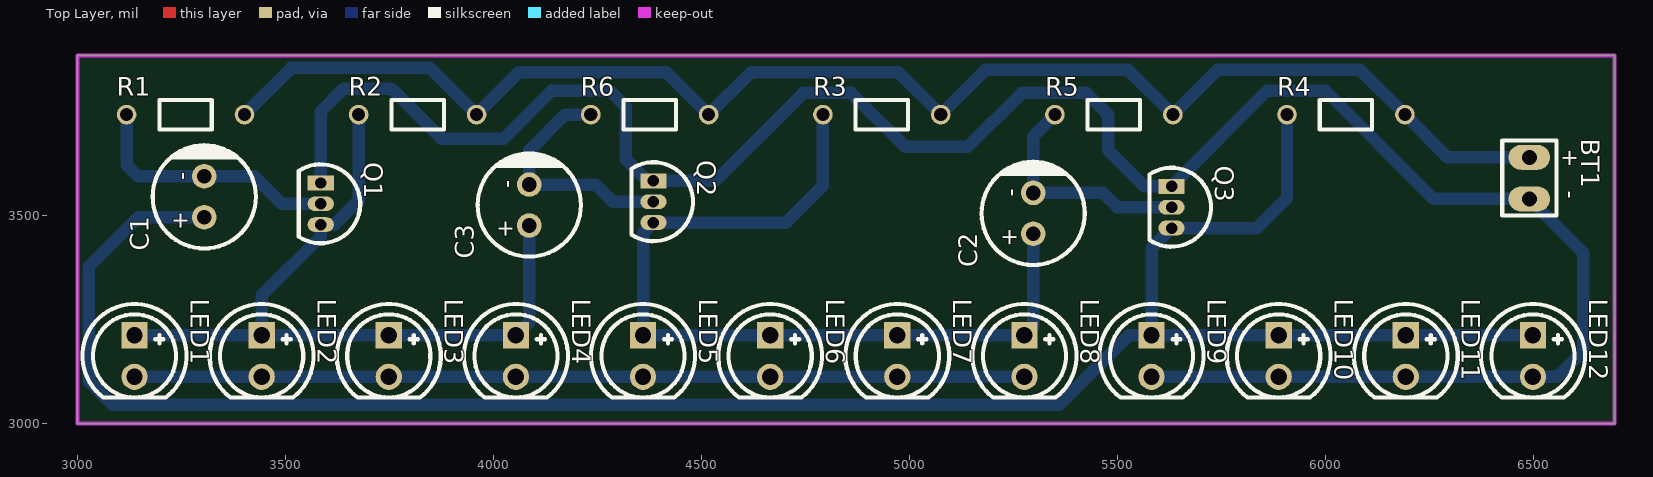
[diagram p0: Top Layer view]
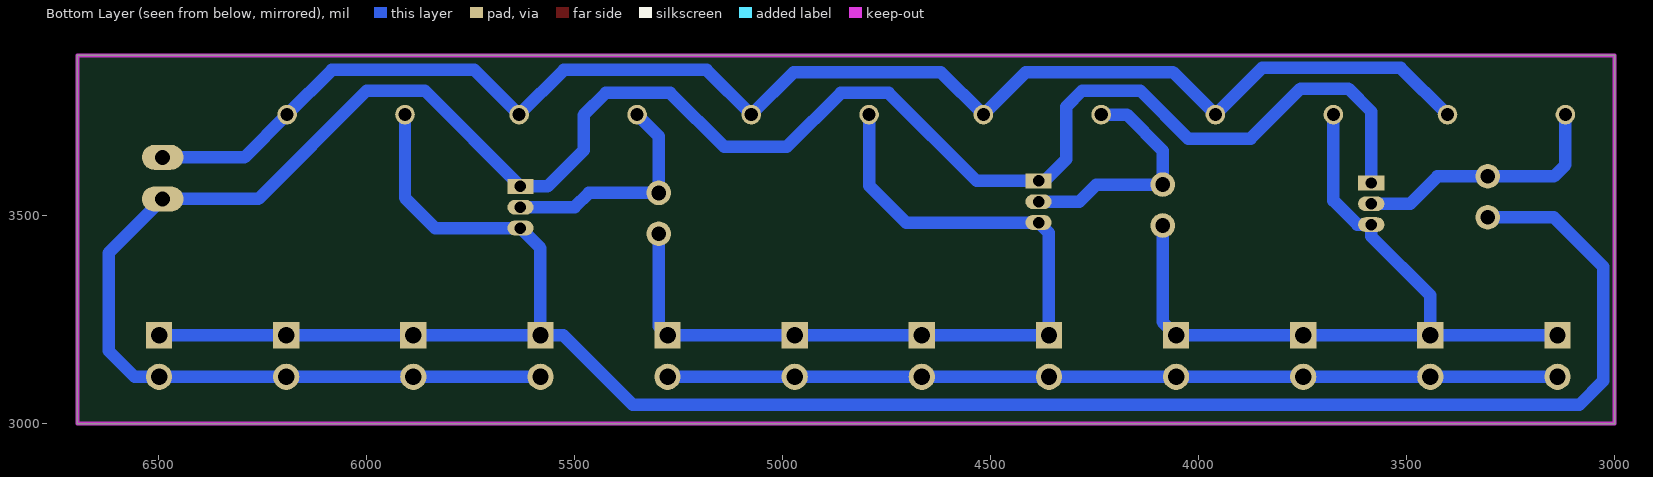
[diagram p1: Bottom Layer view, seen from below]
# Altium PCB MISC75405.pcbdoc
Units mil, origin at the board's own origin, x right, y up, seen from the top; angles counter-clockwise.
Board outline 3695 x 885 mil, 2 copper layers (Top Layer, Bottom Layer), stack 62.206 mil thick; 25 components, 8 nets, 53 pads, 0 vias.

## Layer stack, top to bottom
Top Solder Mask Layer: solder mask 0.394, Dk 3.3
Top Layer: signal copper 1.379
Dielectric1: surface 59.449, FR4, Dk 4.5
Bottom Layer: signal copper 1.378
Bottom Solder Mask Layer: solder mask 0.394, Dk 3.3

## Board outline
3000,3885 3000,3000 6695,3000 6695,3885

## Design rules (kind name [scope] priority, off if disabled: settings)
BoardOutlineClearance copperThickness2oz_1 [All] p2 off: genericclearance=7.99 ignorepadtopadclearanceinfootprint=FALSE except(0: Arc-SplitContinuation Track-SplitContinuation SMDPad-SplitContinuation THPad-SplitContinuation Via-SplitContinuation Fill-SplitContinuation Region-SplitContinuation Poly-SplitContinuation Text-SplitContinuation Hole-SplitContinuation; 5.98: Arc-CutoutEdge SMDPad-CutoutEdge THPad-CutoutEdge Via-CutoutEdge Fill-CutoutEdge Region-CutoutEdge Text-CutoutEdge; 6.93: Hole-OutlineEdge Hole-CutoutEdge; 10: Poly-OutlineEdge Poly-CutoutEdge; 11.81: Arc-OutlineEdge Track-OutlineEdge SMDPad-OutlineEdge THPad-OutlineEdge Via-OutlineEdge Fill-OutlineEdge Region-OutlineEdge Text-OutlineEdge Track-CutoutEdge)
BoardOutlineClearance copperThickness1oz_1 [All] p4: genericclearance=4.02 ignorepadtopadclearanceinfootprint=FALSE except(0: Arc-SplitContinuation Track-SplitContinuation SMDPad-SplitContinuation THPad-SplitContinuation Via-SplitContinuation Fill-SplitContinuation Region-SplitContinuation Poly-SplitContinuation Text-SplitContinuation Hole-SplitContinuation; 6: SMDPad-CutoutEdge THPad-CutoutEdge Via-CutoutEdge Fill-CutoutEdge Region-CutoutEdge Text-CutoutEdge; 6.93: Hole-OutlineEdge Hole-CutoutEdge; 10: Poly-OutlineEdge Poly-CutoutEdge; 11.8: Arc-OutlineEdge Track-OutlineEdge SMDPad-OutlineEdge THPad-OutlineEdge Via-OutlineEdge Fill-OutlineEdge Region-OutlineEdge Text-OutlineEdge; 11.81: Arc-CutoutEdge Track-CutoutEdge)
Clearance copperThickness2oz [All] p1 off: gap=7.99 ignorepadtopadclearanceinfootprint=FALSE except(5.98: SMDPad-Track SMDPad-SMDPad THPad-Track SMDPad-THPad THPad-THPad Track-Via SMDPad-Via THPad-Via Via-Via Fill-Track Region-Track Fill-SMDPad Region-SMDPad Fill-THPad Region-THPad Fill-Via Region-Via Fill-Fill Fill-Region Region-Region Arc-Track Arc-SMDPad Arc-THPad Arc-Via Fill-Arc Region-Arc Arc-Arc Text-Track SMDPad-Text Text-THPad Text-Via Fill-Text Region-Text Arc-Text Text-Text; 6.93: Hole-Track Hole-SMDPad Hole-THPad Hole-Via Fill-Hole Region-Hole Hole-Arc Hole-Text; 10: Poly-Track Poly-SMDPad Poly-THPad Poly-Via Poly-Fill Poly-Region Poly-Poly Poly-Arc Poly-Text Poly-Hole)
Clearance copperThickness1oz [All] p3: gap=4.02 ignorepadtopadclearanceinfootprint=FALSE except(5.98: SMDPad-Track SMDPad-SMDPad THPad-Track SMDPad-THPad THPad-THPad Track-Via SMDPad-Via THPad-Via Via-Via Fill-Track Region-Track Fill-SMDPad Region-SMDPad Fill-THPad Region-THPad Fill-Via Region-Via Fill-Fill Fill-Region Region-Region; 6: Arc-Track Arc-SMDPad Arc-THPad Arc-Via Fill-Arc Region-Arc Arc-Arc Text-Track SMDPad-Text Text-THPad Text-Via Fill-Text Region-Text Arc-Text Text-Text; 6.93: Hole-Track Hole-SMDPad Hole-THPad Hole-Via Fill-Hole Region-Hole Hole-Arc Hole-Text; 10: Poly-Track Poly-SMDPad Poly-THPad Poly-Via Poly-Fill Poly-Region Poly-Poly Poly-Arc Poly-Text Poly-Hole)
DiffPairsRouting differentialPair [All] p1: maxlimit=6 minlimit=6 mostfreqgap=6 toplayer_minwidth=5 toplayer_prefwidth=10 toplayer_maxwidth=100 toplayer_mingap=6 toplayer_prefgap=6 toplayer_maxgap=6 bottomlayer_minwidth=5 bottomlayer_prefwidth=10 bottomlayer_maxwidth=100 bottomlayer_mingap=6 bottomlayer_prefgap=6 bottomlayer_maxgap=6 maxuncoupledlength=10
HoleToHoleClearance otherClearance [All] p1: gap=11.81 allowstackedmicrovias=TRUE
Length netLength [All] p1: minlimit=0 maxlimit=0
MatchedLengths netLengthTolerance [All] p1: tolerance=1000
PasteMaskExpansion pasteMaskExpansion [All] p1: expansion=0
PlaneConnect innerPlane [All] p1: planeconnectstyle=Relief reliefexpansion=20 reliefentries=4 reliefconductorwidth=10 reliefairgap=10
PolygonConnect copperRegion [All] p1: connectstyle=Relief reliefconductorwidth=10 reliefentries=4 polygonreliefangle="90 Angle" airgapwidth=10 via.connectstyle=Relief via.reliefconductorwidth=10 via.reliefentries=4 via.polygonreliefangle="90 Angle" via.airgapwidth=10
RoutingVias viaSize [All] p1: holewidth=12.01 width=24.02 viastyle="Through Hole" minholewidth=11.81 minwidth=19.68 maxholewidth=248.03 maxwidth=393.7
SolderMaskExpansion solderMaskExpansion [IsVia] p1: expansion=-1000 istentingtop=TRUE
SolderMaskExpansion solderMaskExpansion [All] p2: expansion=2 istentingtop=FALSE
Width copperThickness2oz_2 [All] p1 off: maxlimit=100 minlimit=8 preferedwidth=10
Width copperThickness1oz_2 [All] p2: maxlimit=100 minlimit=5 preferedwidth=10

## Components (designator, comment, footprint, x,y, rotation, side; value= is the part's Value field where it differs from the comment)
BT1 "9V battery wire clip Cu 100mm" BAT-TH_2P-9VBATTERY 6490,3590 r270 top
C1 "47uF" CAP-TH_BD6.3-P2.50-D0.5-FD 3305,3545 r90 top
C2 "47uF" CAP-TH_BD6.3-P2.50-D0.5-FD 5297.41,3505.27 r90 top
C3 "47uF" CAP-TH_BD6.3-P2.50-D0.5-FD 4086.19,3525.27 r90 top
LED1 "" LED-TH_5mm 3137.36,3162.51 r270 top
LED2 "" LED-TH_5mm 3442.93,3162.51 r270 top
LED3 "" LED-TH_5mm 3748.5,3162.51 r270 top
LED4 "" LED-TH_5mm 4054.07,3162.51 r270 top
LED5 "" LED-TH_5mm 4359.64,3162.51 r270 top
LED6 "" LED-TH_5mm 4665.21,3162.51 r270 top
LED7 "" LED-TH_5mm 4970.78,3162.51 r270 top
LED8 "" LED-TH_5mm 5276.35,3162.51 r270 top
LED9 "" LED-TH_5mm 5581.92,3162.51 r270 top
LED10 "" LED-TH_5mm 5887.49,3162.51 r270 top
LED11 "" LED-TH_5mm 6193.06,3162.51 r270 top
LED12 "" LED-TH_5mm 6498.63,3162.51 r270 top
Q1 "" S8050_TO_92 3585,3528.25 r270 top
Q2 "" S8050_TO_92 4384.68,3533.25 r270 top
Q3 "" S8050_TO_92 5630,3520 r270 top
R1 "9.1kΩ" Res_1/8W 3260,3740 r0 top
R2 "470" Res_1/8W 3817.84,3740 r0 top
R3 "470" Res_1/8W 4933.53,3740 r0 top
R4 "470" Res_1/8W 6049.22,3740 r0 top
R5 "10kΩ" Res_1/8W 5491.38,3740 r0 top
R6 "10kΩ" Res_1/8W 4375.69,3740 r0 top

## Footprints (in the part's own frame and the unit in brackets; to place one, negate y for a bottom-side part, rotate by r counter-clockwise, add the part's x,y. Pads: shape width x height; smd on the part's side, far side on the other; paste and mask are expansions set on the pad)
BAT-TH_2P-9VBATTERY [mil]
  oval 60x100 hole 36 paste+0 mask+1.97: 1(-50,0) 2(50,0)
  silkscreen extent -90,-65 90,65
CAP-TH_BD6.3-P2.50-D0.5-FD [mm]
  round 1.5 hole 0.9 paste+0 mask+0.05: 1(-1.25,0) 2(1.25,0)
  silkscreen extent -3.15,-3.15 3.21,3.15
LED-TH_5mm [mm]
  rect 1.6x1.6 hole 1 paste+0 mask+0.051: 1(-1.27,0)
  round 1.6 hole 1 paste+0 mask+0.051: 2(1.27,0)
  silkscreen extent -3.17,-3.17 2.54,3.17
Res_1/8W [mil]
  round 47.2 hole 31.5 paste+0 mask+2: 1(-141.7,2.48) 2(141.7,2.48)
  silkscreen extent -63,-33 63,38
S8050_TO_92 [mil]
  rect 35.4x63 hole 27.6 paste+0 mask+2: 1(-50,0)
  oval 35.4x63 hole 27.6 paste+0 mask+2: 2(0,0) 3(50,0)
  silkscreen extent -95,-53 95,95

## Nets (pads, with @x,y where several pads share a name; then routed paths per layer and width w, separated by ;. In a path a pad name is that pad's centre, name@x,y a point inside that pad or via, vN(x,y) a via of type N, cw(c..) or ccw(c..) an arc to the next point about the centre after c; other vN are vias at no path point)
$1N1: C1.2 Q1.2 R1.1 | length 626.2
  Bottom Layer w30: R1.1 3118.3,3621.7 3145.79,3594.21 C1.2 3425.79,3594.21 3491.75,3528.25 Q1.2
$1N2: C3.1 LED1.1 LED2.1 LED3.1 LED4.1 Q1.3 R2.1 | length 1839.6
  Bottom Layer w30: LED1.1 LED2.1 ; R2.1 3676.14,3536.14 3618.25,3478.25 Q1.3 3585,3450 3442.93,3307.93 LED2.1 ; C3.1 4086.19,3244.63 LED4.1 LED3.1 LED2.1
$1N8: C1.1 LED9.1 LED10.1 LED11.1 LED12.1 Q3.3 R4.1 | length 4951.3
  Bottom Layer w30: C1.1 3145.79,3495.79 3026.8,3376.8 3026.8,3103.2 3085,3045 5360,3045 5527.51,3212.51 LED9.1 ; R4.1 5907.52,3542.52 5835,3470 Q3.3 5581.92,3421.92 LED9.1 ; LED12.1 LED11.1 LED10.1 LED9.1
$1N11: BT1.1 R1.2 R2.2 R3.2 R4.2 R5.2 R6.2 | length 3572
  Bottom Layer w30: R1.2 3514.22,3855 3847.02,3855 R2.2 4062.07,3845 4414.87,3845 R6.2 4619.91,3845 4972.71,3845 R3.2 5182.76,3850 5525.55,3850 R5.2 5740.6,3850 6083.4,3850 R4.2 6293.4,3640 BT1.1
$1N12: C2.2 Q3.2 R5.1 | length 556.5
  Bottom Layer w30: R5.1 5297.41,3690.21 C2.2 5465.52,3554.48 5500,3520 Q3.2
$1N15: C3.2 Q2.2 R6.1 | length 580.8
  Bottom Layer w30: R6.1 4172.48,3742.48 4086.19,3656.19 C3.2 4245.52,3574.48 4286.75,3533.25 Q2.2
$1N16: C2.1 LED5.1 LED6.1 LED7.1 LED8.1 Q2.3 R3.1 | length 2064.6
  Bottom Layer w30: R3.1 4791.83,3571.83 4703.25,3483.25 Q2.3 4359.64,3458.21 LED5.1 LED6.1 LED7.1 LED8.1 5297.41,3233.57 C2.1
GND: BT1.2 LED1.2 LED2.2 LED3.2 LED4.2 LED5.2 LED6.2 LED7.2 LED8.2 LED9.2 LED10.2 LED11.2 LED12.2 Q1.1 Q2.1 Q3.1 | length 7523.8
  Bottom Layer w30: LED1.2 LED2.2 LED3.2 LED4.2 LED5.2 LED6.2 LED7.2 LED8.2 ; Q1.1 3585,3750 3640,3805 3755,3805 3875,3685 4025,3685 4140,3800 4280,3800 4318.61,3761.39 4318.61,3635 4370.36,3583.25 Q2.1 4533.25,3583.25 4745,3795 4860,3795 4990,3665 5140,3665 5270,3795 5425,3795 5478.41,3741.59 5478.41,3656.59 5565,3570 Q3.1 5860,3800 6000,3800 6260,3540 BT1.2 6620,3410 6620,3175 6557.51,3112.51 LED12.2 LED11.2 LED10.2 LED9.2

## Keep-outs
Board Outline Layer:
  the board outline again, w10